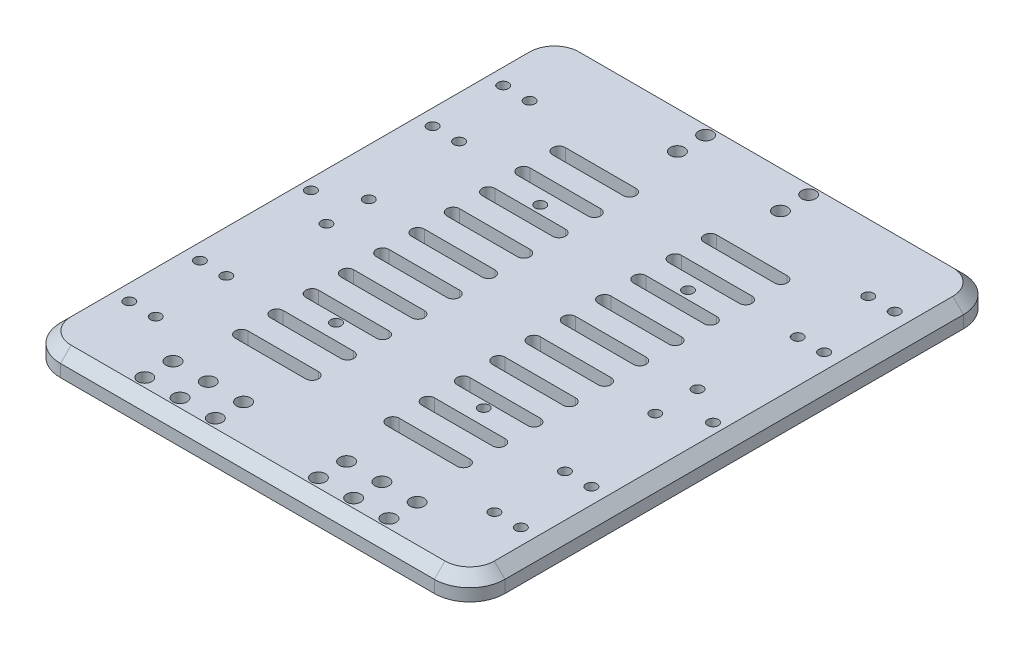
from build123d import *

# Parameters (mm, degrees)
SKETCH1_W               = 126
SKETCH1_H               = 150
BOSS_EXTRUDE1_DEPTH     = 6.5
SKETCH2_R               = 1.5
CUT_EXTRUDE1_DEPTH      = 10
MIRROR2_COPY_1_SKETCH_R = 1.5
MIRROR2_COPY_1_DEPTH    = 10
FILLET1_R               = 10
SKETCH4_R               = 1.5
CUT_EXTRUDE3_DEPTH      = 10
SKETCH5_R               = 2
CUT_EXTRUDE4_DEPTH      = 20
MIRROR5_COPY_1_SKETCH_R = 2
MIRROR5_COPY_1_DEPTH    = 20
SKETCH6_R               = 2
CUT_EXTRUDE5_DEPTH      = 99.164402917
CUT_EXTRUDE6_DEPTH      = 99.164402917
CHAMFER1_SIZE           = 3
SKETCH8_R               = 1.5
CUT_EXTRUDE7_DEPTH      = 99.164402917


with BuildPart() as part:
    # Sketch1 → Boss-Extrude1 (new body)
    with BuildSketch(Plane(origin=(0, 0, 0), x_dir=(1, 0, 0), z_dir=(0, 1, 0))):
        Rectangle(SKETCH1_W, SKETCH1_H)
    extrude(amount=BOSS_EXTRUDE1_DEPTH)

    # Sketch2 → Cut-Extrude1 (cut)
    with BuildSketch(Plane(origin=(0, 6.5, 0), x_dir=(1, 0, 0), z_dir=(0, 1, 0))):
        with Locations(Location((-55.5, 33, 0), (0, 0, 270))):
            Circle(SKETCH2_R)
        with Locations(Location((-48, 33, 0), (0, 0, 90))):
            Circle(SKETCH2_R)
        with Locations(Location((-48, 53, 0), (0, 0, 270))):
            Circle(SKETCH2_R)
        with Locations(Location((-55.5, 53, 0), (0, 0, 90))):
            Circle(SKETCH2_R)
    cut_extrude1 = extrude(amount=-CUT_EXTRUDE1_DEPTH, mode=Mode.SUBTRACT)

    # Mirror1: Cut-Extrude1 across plane
    add(cut_extrude1.mirror(Plane(origin=(0, 0, 0), x_dir=(0, 0, 1), z_dir=(1, 0, 0))), mode=Mode.SUBTRACT)

    # Mirror2: Cut-Extrude1 across plane
    add(cut_extrude1.mirror(Plane.XY), mode=Mode.SUBTRACT)

    # Mirror2 copy 1 sketch → Mirror2 copy 1 (cut)
    with BuildSketch(Plane(origin=(0, 6.5, 0), x_dir=(-1, 0, 0), z_dir=(0, 1, 0))):
        with Locations(Location((-55.5, 33, 0), (0, 0, 270))):
            Circle(MIRROR2_COPY_1_SKETCH_R)
        with Locations(Location((-48, 33, 0), (0, 0, 90))):
            Circle(MIRROR2_COPY_1_SKETCH_R)
        with Locations(Location((-48, 53, 0), (0, 0, 270))):
            Circle(MIRROR2_COPY_1_SKETCH_R)
        with Locations(Location((-55.5, 53, 0), (0, 0, 90))):
            Circle(MIRROR2_COPY_1_SKETCH_R)
    extrude(amount=-MIRROR2_COPY_1_DEPTH, mode=Mode.SUBTRACT)

    # Fillet1
    fillet1_edges = [part.edges().sort_by_distance(p)[0] for p in [
        (63, 3.25, 75),
        (-63, 3.25, 75),
        (-63, 3.25, -75),
        (63, 3.25, -75),
    ]]
    fillet(fillet1_edges, radius=FILLET1_R)

    # Sketch4 → Cut-Extrude3 (cut)
    with BuildSketch(Plane(origin=(0, 6.5, 0), x_dir=(1, 0, 0), z_dir=(0, 1, 0))):
        with Locations(Location((-46.607695155, -6, 0), (0, 0, 270))):
            Circle(SKETCH4_R)
        with Locations(Location((-46.607695155, 6, 0), (0, 0, 270))):
            Circle(SKETCH4_R)
        with Locations(Location((-57, 0, 0), (0, 0, 270))):
            Circle(SKETCH4_R)
    cut_extrude3 = extrude(amount=-CUT_EXTRUDE3_DEPTH, mode=Mode.SUBTRACT)

    # Mirror3: Cut-Extrude3 across plane
    add(cut_extrude3.mirror(Plane(origin=(0, 0, 0), x_dir=(0, 0, 1), z_dir=(1, 0, 0))), mode=Mode.SUBTRACT)

    # Sketch5 → Cut-Extrude4 (cut)
    with BuildSketch(Plane(origin=(0, 6.5, 0), x_dir=(1, 0, 0), z_dir=(0, 1, 0))):
        with Locations(Location((14.61, -61.5, 0), (0, 0, 270))):
            Circle(SKETCH5_R)
        with Locations(Location((14.61, -69.5, 0), (0, 0, 270))):
            Circle(SKETCH5_R)
    cut_extrude4 = extrude(amount=-CUT_EXTRUDE4_DEPTH, mode=Mode.SUBTRACT)

    # Mirror4: Cut-Extrude4 across plane
    add(cut_extrude4.mirror(Plane(origin=(0, 0, 0), x_dir=(0, 0, 1), z_dir=(1, 0, 0))), mode=Mode.SUBTRACT)

    # Mirror5: Cut-Extrude4 across plane
    add(cut_extrude4.mirror(Plane.XY), mode=Mode.SUBTRACT)

    # Mirror5 copy 1 sketch → Mirror5 copy 1 (cut)
    with BuildSketch(Plane(origin=(0, 6.5, 0), x_dir=(-1, 0, 0), z_dir=(0, 1, 0))):
        with Locations(Location((14.61, -61.5, 0), (0, 0, 270))):
            Circle(MIRROR5_COPY_1_SKETCH_R)
        with Locations(Location((14.61, -69.5, 0), (0, 0, 270))):
            Circle(MIRROR5_COPY_1_SKETCH_R)
    extrude(amount=-MIRROR5_COPY_1_DEPTH, mode=Mode.SUBTRACT)

    # Sketch6 → Cut-Extrude5 (cut, through all)
    with BuildSketch(Plane(origin=(0, 6.5, 0), x_dir=(1, 0, 0), z_dir=(0, 1, 0))):
        with Locations(Location((14.61, -69.5, 0), (0, 0, 270))):
            Circle(SKETCH6_R)
        with Locations(Location((14.61, -61.5, 0), (0, 0, 270))):
            Circle(SKETCH6_R)
        with Locations(Location((24.61, -61.5, 0), (0, 0, 270))):
            Circle(SKETCH6_R)
        with Locations(Location((24.61, -69.5, 0), (0, 0, 270))):
            Circle(SKETCH6_R)
        with Locations(Location((34.61, -61.5, 0), (0, 0, 270))):
            Circle(SKETCH6_R)
        with Locations(Location((34.61, -69.5, 0), (0, 0, 270))):
            Circle(SKETCH6_R)
        with Locations(Location((-14.61, -61.5, 0), (0, 0, 270))):
            Circle(SKETCH6_R)
        with Locations(Location((-14.61, -69.5, 0), (0, 0, 270))):
            Circle(SKETCH6_R)
        with Locations(Location((-24.61, -61.5, 0), (0, 0, 270))):
            Circle(SKETCH6_R)
        with Locations(Location((-24.61, -69.5, 0), (0, 0, 270))):
            Circle(SKETCH6_R)
        with Locations(Location((-34.61, -61.5, 0), (0, 0, 270))):
            Circle(SKETCH6_R)
        with Locations(Location((-34.61, -69.5, 0), (0, 0, 270))):
            Circle(SKETCH6_R)
    extrude(amount=-CUT_EXTRUDE5_DEPTH, mode=Mode.SUBTRACT)

    # Sketch7 → Cut-Extrude6 (cut, through all)
    with BuildSketch(Plane(origin=(0, 6.5, 0), x_dir=(1, 0, 0), z_dir=(0, 1, 0))):
        with BuildLine():
            Line((-31.451375683, 46.57548811), (-11.451375683, 46.57548811))
            ThreePointArc((-11.451375683, 46.57548811), (-9.654719619, 44.778832046), (-11.451375683, 42.982175982))
            Line((-11.451375683, 42.982175982), (-31.451375683, 42.982175982))
            ThreePointArc((-31.451375683, 42.982175982), (-33.248031746, 44.778832046), (-31.451375683, 46.57548811))
        make_face()
        with BuildLine():
            Line((-31.451375683, 36.57548811), (-11.451375683, 36.57548811))
            ThreePointArc((-11.451375683, 36.57548811), (-9.654719619, 34.778832046), (-11.451375683, 32.982175982))
            Line((-11.451375683, 32.982175982), (-31.451375683, 32.982175982))
            ThreePointArc((-31.451375683, 32.982175982), (-33.248031746, 34.778832046), (-31.451375683, 36.57548811))
        make_face()
        with BuildLine():
            Line((-31.451375683, 26.57548811), (-11.451375683, 26.57548811))
            ThreePointArc((-11.451375683, 26.57548811), (-9.654719619, 24.778832046), (-11.451375683, 22.982175982))
            Line((-11.451375683, 22.982175982), (-31.451375683, 22.982175982))
            ThreePointArc((-31.451375683, 22.982175982), (-33.248031746, 24.778832046), (-31.451375683, 26.57548811))
        make_face()
        with BuildLine():
            Line((-31.451375683, 16.57548811), (-11.451375683, 16.57548811))
            ThreePointArc((-11.451375683, 16.57548811), (-9.654719619, 14.778832046), (-11.451375683, 12.982175982))
            Line((-11.451375683, 12.982175982), (-31.451375683, 12.982175982))
            ThreePointArc((-31.451375683, 12.982175982), (-33.248031746, 14.778832046), (-31.451375683, 16.57548811))
        make_face()
        with BuildLine():
            Line((-31.451375683, 6.57548811), (-11.451375683, 6.57548811))
            ThreePointArc((-11.451375683, 6.57548811), (-9.654719619, 4.778832046), (-11.451375683, 2.982175982))
            Line((-11.451375683, 2.982175982), (-31.451375683, 2.982175982))
            ThreePointArc((-31.451375683, 2.982175982), (-33.248031746, 4.778832046), (-31.451375683, 6.57548811))
        make_face()
        with BuildLine():
            Line((-31.451375683, -3.42451189), (-11.451375683, -3.42451189))
            ThreePointArc((-11.451375683, -3.42451189), (-9.654719619, -5.221167954), (-11.451375683, -7.017824018))
            Line((-11.451375683, -7.017824018), (-31.451375683, -7.017824018))
            ThreePointArc((-31.451375683, -7.017824018), (-33.248031746, -5.221167954), (-31.451375683, -3.42451189))
        make_face()
        with BuildLine():
            Line((-31.451375683, -13.42451189), (-11.451375683, -13.42451189))
            ThreePointArc((-11.451375683, -13.42451189), (-9.654719619, -15.221167954), (-11.451375683, -17.017824018))
            Line((-11.451375683, -17.017824018), (-31.451375683, -17.017824018))
            ThreePointArc((-31.451375683, -17.017824018), (-33.248031746, -15.221167954), (-31.451375683, -13.42451189))
        make_face()
        with BuildLine():
            Line((-31.451375683, -23.42451189), (-11.451375683, -23.42451189))
            ThreePointArc((-11.451375683, -23.42451189), (-9.654719619, -25.221167954), (-11.451375683, -27.017824018))
            Line((-11.451375683, -27.017824018), (-31.451375683, -27.017824018))
            ThreePointArc((-31.451375683, -27.017824018), (-33.248031746, -25.221167954), (-31.451375683, -23.42451189))
        make_face()
        with BuildLine():
            Line((-31.451375683, -33.42451189), (-11.451375683, -33.42451189))
            ThreePointArc((-11.451375683, -33.42451189), (-9.654719619, -35.221167954), (-11.451375683, -37.017824018))
            Line((-11.451375683, -37.017824018), (-31.451375683, -37.017824018))
            ThreePointArc((-31.451375683, -37.017824018), (-33.248031746, -35.221167954), (-31.451375683, -33.42451189))
        make_face()
        with BuildLine():
            Line((-31.451375683, -43.42451189), (-11.451375683, -43.42451189))
            ThreePointArc((-11.451375683, -43.42451189), (-9.654719619, -45.221167954), (-11.451375683, -47.017824018))
            Line((-11.451375683, -47.017824018), (-31.451375683, -47.017824018))
            ThreePointArc((-31.451375683, -47.017824018), (-33.248031746, -45.221167954), (-31.451375683, -43.42451189))
        make_face()
        with BuildLine():
            Line((31.451375683, 46.57548811), (11.451375683, 46.57548811))
            ThreePointArc((11.451375683, 46.57548811), (9.654719619, 44.778832046), (11.451375683, 42.982175982))
            Line((11.451375683, 42.982175982), (31.451375683, 42.982175982))
            ThreePointArc((31.451375683, 42.982175982), (33.248031746, 44.778832046), (31.451375683, 46.57548811))
        make_face()
        with BuildLine():
            Line((31.451375683, 36.57548811), (11.451375683, 36.57548811))
            ThreePointArc((11.451375683, 36.57548811), (9.654719619, 34.778832046), (11.451375683, 32.982175982))
            Line((11.451375683, 32.982175982), (31.451375683, 32.982175982))
            ThreePointArc((31.451375683, 32.982175982), (33.248031746, 34.778832046), (31.451375683, 36.57548811))
        make_face()
        with BuildLine():
            Line((31.451375683, 26.57548811), (11.451375683, 26.57548811))
            ThreePointArc((11.451375683, 26.57548811), (9.654719619, 24.778832046), (11.451375683, 22.982175982))
            Line((11.451375683, 22.982175982), (31.451375683, 22.982175982))
            ThreePointArc((31.451375683, 22.982175982), (33.248031746, 24.778832046), (31.451375683, 26.57548811))
        make_face()
        with BuildLine():
            Line((31.451375683, 16.57548811), (11.451375683, 16.57548811))
            ThreePointArc((11.451375683, 16.57548811), (9.654719619, 14.778832046), (11.451375683, 12.982175982))
            Line((11.451375683, 12.982175982), (31.451375683, 12.982175982))
            ThreePointArc((31.451375683, 12.982175982), (33.248031746, 14.778832046), (31.451375683, 16.57548811))
        make_face()
        with BuildLine():
            Line((31.451375683, 6.57548811), (11.451375683, 6.57548811))
            ThreePointArc((11.451375683, 6.57548811), (9.654719619, 4.778832046), (11.451375683, 2.982175982))
            Line((11.451375683, 2.982175982), (31.451375683, 2.982175982))
            ThreePointArc((31.451375683, 2.982175982), (33.248031746, 4.778832046), (31.451375683, 6.57548811))
        make_face()
        with BuildLine():
            Line((31.451375683, -3.42451189), (11.451375683, -3.42451189))
            ThreePointArc((11.451375683, -3.42451189), (9.654719619, -5.221167954), (11.451375683, -7.017824018))
            Line((11.451375683, -7.017824018), (31.451375683, -7.017824018))
            ThreePointArc((31.451375683, -7.017824018), (33.248031746, -5.221167954), (31.451375683, -3.42451189))
        make_face()
        with BuildLine():
            Line((31.451375683, -13.42451189), (11.451375683, -13.42451189))
            ThreePointArc((11.451375683, -13.42451189), (9.654719619, -15.221167954), (11.451375683, -17.017824018))
            Line((11.451375683, -17.017824018), (31.451375683, -17.017824018))
            ThreePointArc((31.451375683, -17.017824018), (33.248031746, -15.221167954), (31.451375683, -13.42451189))
        make_face()
        with BuildLine():
            Line((31.451375683, -23.42451189), (11.451375683, -23.42451189))
            ThreePointArc((11.451375683, -23.42451189), (9.654719619, -25.221167954), (11.451375683, -27.017824018))
            Line((11.451375683, -27.017824018), (31.451375683, -27.017824018))
            ThreePointArc((31.451375683, -27.017824018), (33.248031746, -25.221167954), (31.451375683, -23.42451189))
        make_face()
        with BuildLine():
            Line((31.451375683, -33.42451189), (11.451375683, -33.42451189))
            ThreePointArc((11.451375683, -33.42451189), (9.654719619, -35.221167954), (11.451375683, -37.017824018))
            Line((11.451375683, -37.017824018), (31.451375683, -37.017824018))
            ThreePointArc((31.451375683, -37.017824018), (33.248031746, -35.221167954), (31.451375683, -33.42451189))
        make_face()
        with BuildLine():
            Line((31.451375683, -43.42451189), (11.451375683, -43.42451189))
            ThreePointArc((11.451375683, -43.42451189), (9.654719619, -45.221167954), (11.451375683, -47.017824018))
            Line((11.451375683, -47.017824018), (31.451375683, -47.017824018))
            ThreePointArc((31.451375683, -47.017824018), (33.248031746, -45.221167954), (31.451375683, -43.42451189))
        make_face()
    extrude(amount=-CUT_EXTRUDE6_DEPTH, mode=Mode.SUBTRACT)

    # Chamfer1
    chamfer1_edges = [part.edges().sort_by_distance(p)[0] for p in [
        (0, 6.5, 75),
        (0, 6.5, -75),
        (-63, 6.5, 0),
        (-60.071067812, 6.5, -72.071067812),
        (60.071067812, 6.5, -72.071067812),
        (-60.071067812, 6.5, 72.071067812),
        (60.071067812, 6.5, 72.071067812),
        (63, 6.5, 0),
    ]]
    chamfer(chamfer1_edges, length=CHAMFER1_SIZE)

    # Sketch8 → Cut-Extrude7 (cut, through all)
    with BuildSketch(Plane.XZ):
        with Locations(Location((20.95, -28.95, 0), (0, 0, 270))):
            Circle(SKETCH8_R)
        with Locations(Location((-20.95, -28.95, 0), (0, 0, 270))):
            Circle(SKETCH8_R)
        with Locations(Location((20.95, 28.95, 0), (0, 0, 270))):
            Circle(SKETCH8_R)
        with Locations(Location((-20.95, 28.95, 0), (0, 0, 270))):
            Circle(SKETCH8_R)
    extrude(amount=-CUT_EXTRUDE7_DEPTH, mode=Mode.SUBTRACT)


solid = part.part
